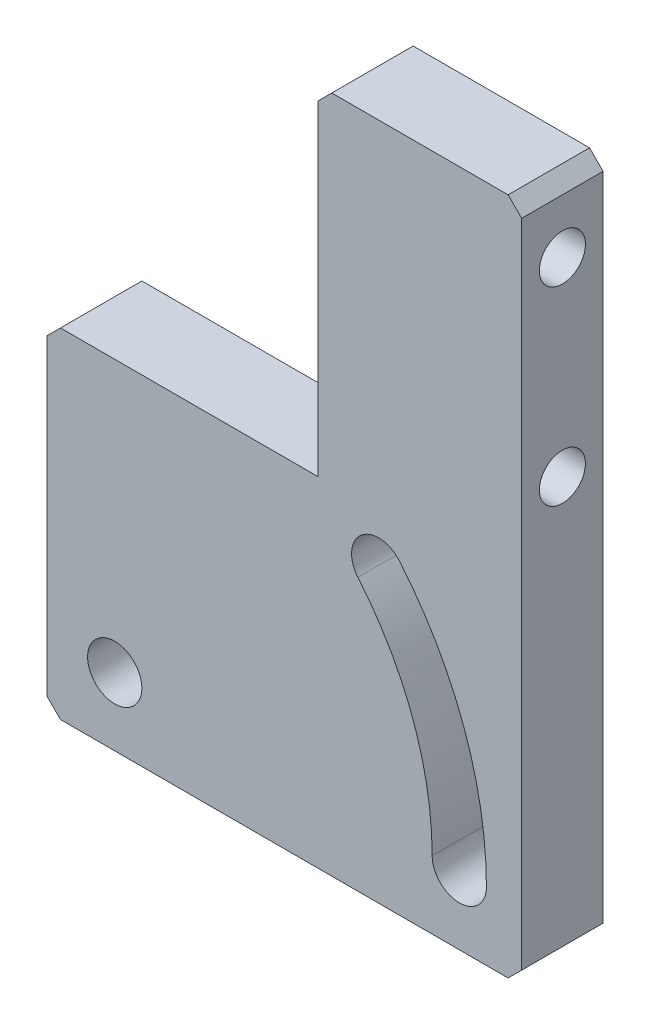
from build123d import *

# Parameters (mm, degrees)
SKETCH_1_W          = 35
SKETCH_1_H          = 50
EXTRUDE_1_DEPTH     = 3
SKETCH_2_W          = 20
SKETCH_2_H          = 25
CUT_EXTRUDE_1_DEPTH = 32.10064308
SKETCH_3_R          = 2
CUT_EXTRUDE_2_DEPTH = 32.10064308
HOLE_WIZARD_M3_1_D  = 3.4
CHAMFER_1_SIZE      = 1


with BuildPart() as part:
    # 草图1 → 凸台-拉伸1 (new, symmetric)
    with BuildSketch(Plane.XY):
        Rectangle(SKETCH_1_W, SKETCH_1_H)
    extrude(amount=EXTRUDE_1_DEPTH, both=True)

    # 草图2 → 切除-拉伸1 (cut, through all)
    with BuildSketch(Plane.XY.offset(3)):
        with Locations((-7.5, 12.5)):
            Rectangle(SKETCH_2_W, SKETCH_2_H)
    extrude(amount=-CUT_EXTRUDE_1_DEPTH, mode=Mode.SUBTRACT)

    # 草图3 → 切除-拉伸2 (cut, through all)
    with BuildSketch(Plane.XY.offset(3)):
        with Locations((-12.5, -20)):
            Circle(SKETCH_3_R)
        with BuildLine():
            ThreePointArc((14.9, -20), (13.24757781, -10.628648073), (8.489617741, -2.387619495))
            ThreePointArc((8.489617741, -2.387619495), (5.671953636, -2.141105828), (5.425439969, -4.958769933))
            ThreePointArc((5.425439969, -4.958769933), (9.488807326, -11.996728646), (10.9, -20))
            ThreePointArc((10.9, -20), (12.9, -22), (14.9, -20))
        make_face()
    extrude(amount=-CUT_EXTRUDE_2_DEPTH, mode=Mode.SUBTRACT)

    # M3 间隙孔1 (through all)
    with Locations(Plane.ZY.offset(-2.5)):
        with Locations((0, 20), (0, 6)):
            Hole(HOLE_WIZARD_M3_1_D / 2)

    # 倒角1
    chamfer_1_edges = [part.edges().sort_by_distance(p)[0] for p in [
        (-17.5, 0, 0),
        (2.5, 25, 0),
        (17.5, 25, 0),
        (17.5, -25, 0),
        (-17.5, -25, 0),
    ]]
    chamfer(chamfer_1_edges, length=CHAMFER_1_SIZE)


solid = part.part
